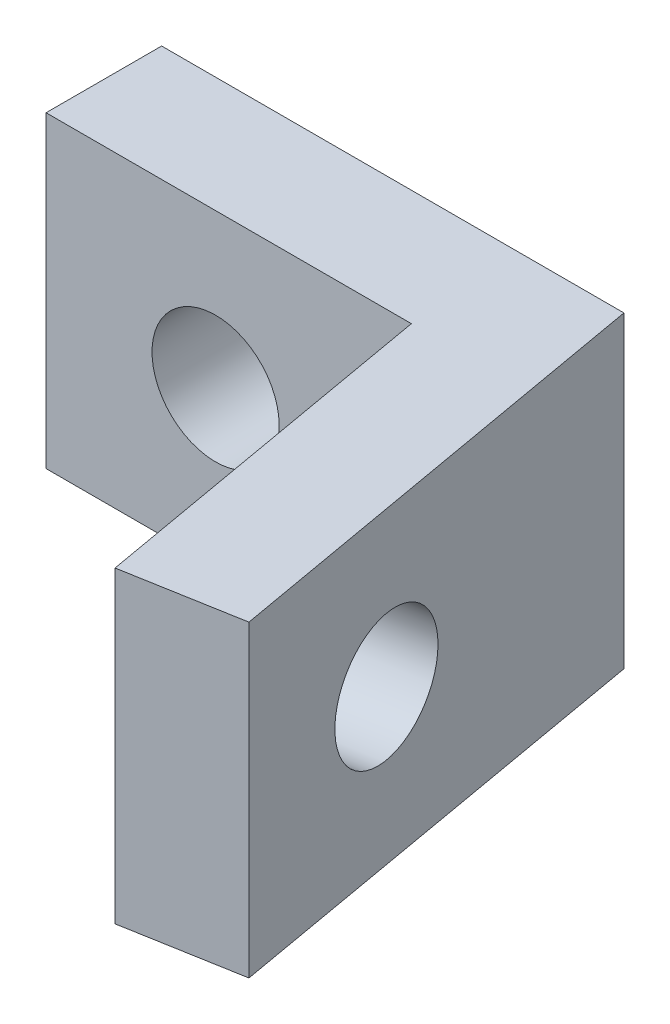
from build123d import *

# Parameters (mm, degrees)
SKETCH_1_W          = 12
SKETCH_1_H          = 8
EXTRUDE_1_DEPTH     = 3
EXTRUDE_2_DEPTH     = 8
SKETCH_3_R          = 1.65
CUT_EXTRUDE_1_DEPTH = 3
SKETCH_4_R          = 1.65
CUT_EXTRUDE_2_DEPTH = 3


with BuildPart() as part:
    # 草图1 → 凸台-拉伸1 (new body)
    with BuildSketch(Plane.XY):
        with Locations((-1.4, 0)):
            Rectangle(SKETCH_1_W, SKETCH_1_H)
    extrude(amount=EXTRUDE_1_DEPTH)

    # 草图2 → 凸台-拉伸2 (add)
    with BuildSketch(Plane.XZ.offset(4)):
        Polygon((4.6, 0), (6.683778132, 11.817693036), (3.729354873, 12.338637569), (2.082701106, 3), align=None)
    extrude(amount=-EXTRUDE_2_DEPTH)

    # 草图3 → 切除-拉伸1 (cut)
    with BuildSketch(Plane.XY.offset(3)):
        with Locations((-3, 0)):
            Circle(SKETCH_3_R)
    extrude(amount=-CUT_EXTRUDE_1_DEPTH, mode=Mode.SUBTRACT)

    # 草图4 → 切除-拉伸2 (cut)
    with BuildSketch(Plane(origin=(4.461293028, 0, -0.78664633), x_dir=(-0.1736481776669236, 0, -0.9848077530122092), z_dir=(0.9848077530122092, 0, -0.1736481776669236))):
        with Locations((-8.398781617, 0)):
            Circle(SKETCH_4_R)
    extrude(amount=-CUT_EXTRUDE_2_DEPTH, mode=Mode.SUBTRACT)


solid = part.part
